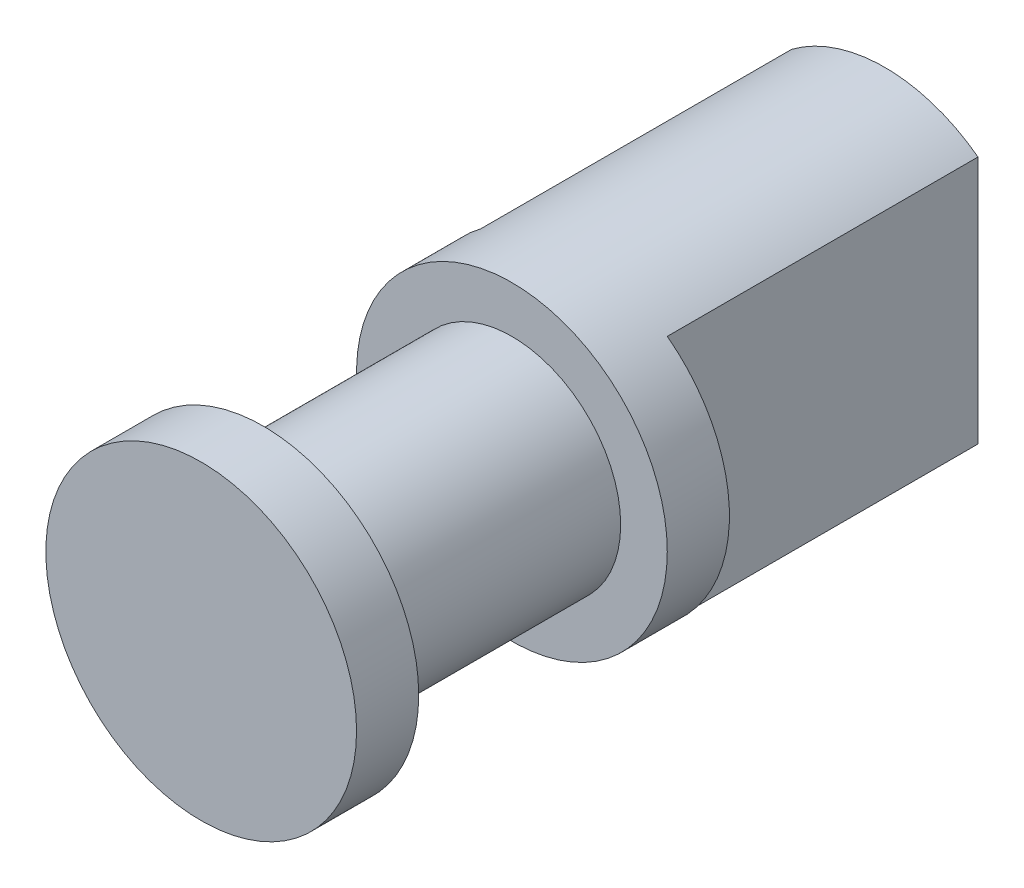
from build123d import *

# Parameters (mm, degrees)
SKETCH1_R           = 2.5
BOSS_EXTRUDE1_DEPTH = 11
SKETCH2_OUTSIDE_W   = 9.616
SKETCH2_OUTSIDE_H   = 9.616
CUT_EXTRUDE1_DEPTH  = 5
CUT_EXTRUDE2_START  = -5
SKETCH3_R           = 2.5
SKETCH3_R_2         = 1.75
CUT_EXTRUDE2_DEPTH  = 4


with BuildPart() as part:
    # Sketch1 → Boss-Extrude1 (new body)
    with BuildSketch(Plane.XY):
        Circle(SKETCH1_R)
    extrude(amount=BOSS_EXTRUDE1_DEPTH)

    # Sketch2 outside → Cut-Extrude1 (cut)
    with BuildSketch(Plane(origin=(0, 0, 0), x_dir=(-1, 0, 0), z_dir=(0, 0, -1))):
        Rectangle(SKETCH2_OUTSIDE_W, SKETCH2_OUTSIDE_H)
        with BuildLine():
            Line((-1.5, 2), (-1.5, -2))
            ThreePointArc((-1.5, -2), (0, -2.5), (1.5, -2))
            Line((1.5, -2), (1.5, 2))
            ThreePointArc((1.5, 2), (0, 2.5), (-1.5, 2))
        make_face(mode=Mode.SUBTRACT)
    extrude(amount=-CUT_EXTRUDE1_DEPTH, mode=Mode.SUBTRACT)

    # Sketch3 → Cut-Extrude2 (cut)
    with BuildSketch(Plane.XY.offset(11).offset(CUT_EXTRUDE2_START)):
        with Locations(Location((0, 0, 0), (0, 0, 126.869897646))):
            Circle(SKETCH3_R)
        Circle(SKETCH3_R_2, mode=Mode.SUBTRACT)
    extrude(amount=CUT_EXTRUDE2_DEPTH, mode=Mode.SUBTRACT)


solid = part.part
